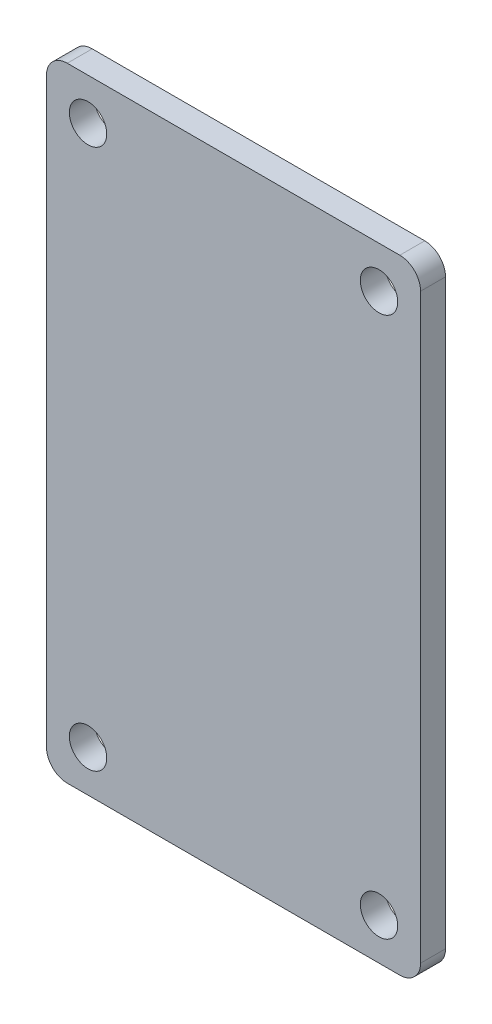
from build123d import *

# Parameters (mm, degrees)
EXTRUDE1_DEPTH = 6
SKETCH2_R      = 9
EXTRUDE2_DEPTH = 176.339670354


with BuildPart() as part:
    # Sketch1 → Extrude1 (new, symmetric)
    with BuildSketch(Plane.XY):
        with BuildLine():
            Line((80, 150), (-80, 150))
            ThreePointArc((-80, 150), (-87.071067812, 147.071067812), (-90, 140))
            Line((-90, 140), (-90, -140))
            ThreePointArc((-90, -140), (-87.071067812, -147.071067812), (-80, -150))
            Line((-80, -150), (80, -150))
            ThreePointArc((80, -150), (87.071067812, -147.071067812), (90, -140))
            Line((90, -140), (90, 140))
            ThreePointArc((90, 140), (87.071067812, 147.071067812), (80, 150))
        make_face()
    extrude(amount=EXTRUDE1_DEPTH, both=True)

    # Sketch2 → Extrude2 (cut, through all)
    with BuildSketch(Plane.XY.offset(6)):
        with Locations((-70, -130)):
            Circle(SKETCH2_R)
        with Locations((70, -130)):
            Circle(SKETCH2_R)
        with Locations((-70, 130)):
            Circle(SKETCH2_R)
        with Locations((70, 130)):
            Circle(SKETCH2_R)
    extrude(amount=-EXTRUDE2_DEPTH, mode=Mode.SUBTRACT)


solid = part.part
